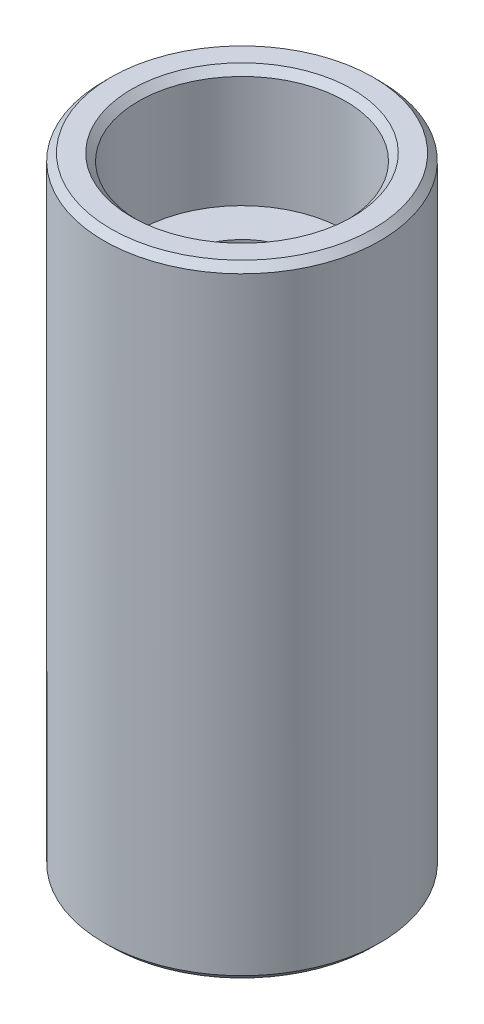
SolidWorks part; units mm, degrees
material "45"
ref_plane "Front Plane" through (0, 0, 0) normal (0, 0, 1) x (1, 0, 0)
ref_plane "Top Plane" through (0, 0, 0) normal (0, 1, 0) x (1, 0, 0)
ref_plane "Right Plane" through (0, 0, 0) normal (1, 0, 0) x (0, 0, -1)
sketch "Sketch1" plane through (0, 0, 0) normal (0, 1, 0) x (1, 0, 0)
  circle A0 centre (0, 0) radius 10
  dimension "D1" = 20
extrude "Boss-Extrude1" add sketch "Sketch1" along normal blind 45
hole_wizard "CBORE for M8 Hex Socket Head Cap Screw1" positions "Sketch5" profile "Sketch4" counterbore size "M8" standard "Iso" end condition through all
sketch "Sketch5" plane through (0, 45, 0) normal (0, 1, 0) x (1, 0, 0)
  point P0 (0, 0)
sketch "Sketch4" plane through (0, 45, 0) normal (1, 0, 0) x (0, 0, 1)
  line L0 (0, 0) -> (0, 45)
  line L1 (0, 45) -> (4.5, 45)
  line L3 (4.5, 45) -> (4.5, 8.6)
  line L4 (4.5, 8.6) -> (7.5, 8.6)
  line L5 (7.5, 8.6) -> (7.5, 0)
  line L7 (7.5, 0) -> (0, 0)
  line L11 (0, -6.35) -> (0, 107.95) construction
  dimension "通孔孔直径" = 9
  dimension "通孔孔深度" = 45
  dimension "柱形沉头孔直径" = 15
  dimension "柱形沉头孔深度" = 8.6
chamfer "Chamfer1" distance 0.5 angle 45 4 edges at (0, 45, 10) (0, 45, 7.5) (0, 0, 10) (0, 0, 4.5)
